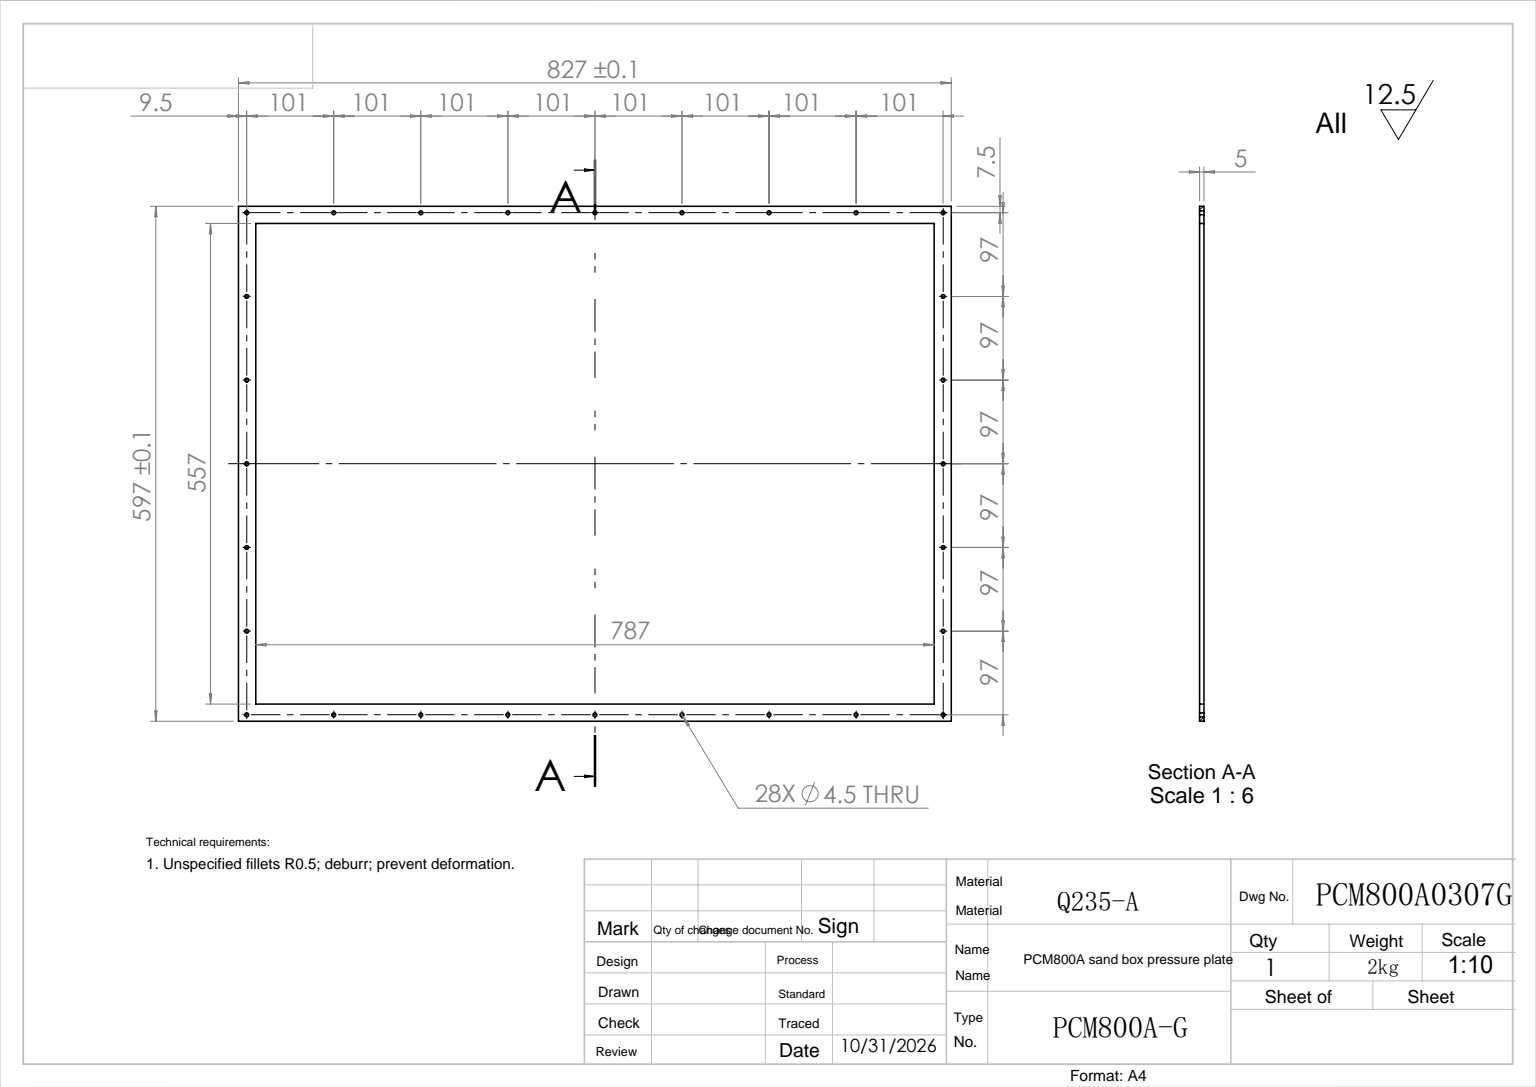
from build123d import *

# Parameters (mm, degrees)
SKETCH_1_W                        = 827
SKETCH_1_H                        = 597
SKETCH_1_W_2                      = 787
SKETCH_1_H_2                      = 557
EXTRUDE_1_DEPTH                   = 5
SKETCH_2_R                        = 2.25
CUT_EXTRUDE_1_DEPTH               = 5
PATTERN_LINEAR_1_COUNT            = 9
PATTERN_LINEAR_1_PITCH            = 101
PATTERN_LINEAR_2_COUNT            = 7
PATTERN_LINEAR_2_PITCH            = 97
PATTERN_LINEAR_3_COPY_1_SKETCH_R  = 2.25
PATTERN_LINEAR_3_COPY_1_DEPTH     = 5
PATTERN_LINEAR_3_COPY_2_SKETCH_R  = 2.25
PATTERN_LINEAR_3_COPY_2_DEPTH     = 5
PATTERN_LINEAR_3_COPY_3_SKETCH_R  = 2.25
PATTERN_LINEAR_3_COPY_3_DEPTH     = 5
PATTERN_LINEAR_3_COPY_4_SKETCH_R  = 2.25
PATTERN_LINEAR_3_COPY_4_DEPTH     = 5
PATTERN_LINEAR_3_COPY_5_SKETCH_R  = 2.25
PATTERN_LINEAR_3_COPY_5_DEPTH     = 5
PATTERN_LINEAR_3_COPY_6_SKETCH_R  = 2.25
PATTERN_LINEAR_3_COPY_6_DEPTH     = 5
PATTERN_LINEAR_3_COPY_7_SKETCH_R  = 2.25
PATTERN_LINEAR_3_COPY_7_DEPTH     = 5
PATTERN_LINEAR_3_COPY_8_SKETCH_R  = 2.25
PATTERN_LINEAR_3_COPY_8_DEPTH     = 5
PATTERN_LINEAR_3_COPY_9_SKETCH_R  = 2.25
PATTERN_LINEAR_3_COPY_9_DEPTH     = 5
PATTERN_LINEAR_3_COPY_10_SKETCH_R = 2.25
PATTERN_LINEAR_3_COPY_10_DEPTH    = 5
PATTERN_LINEAR_3_COPY_11_SKETCH_R = 2.25
PATTERN_LINEAR_3_COPY_11_DEPTH    = 5
PATTERN_LINEAR_3_COPY_12_SKETCH_R = 2.25
PATTERN_LINEAR_3_COPY_12_DEPTH    = 5
PATTERN_LINEAR_3_COPY_13_SKETCH_R = 2.25
PATTERN_LINEAR_3_COPY_13_DEPTH    = 5
PATTERN_LINEAR_3_COPY_14_SKETCH_R = 2.25
PATTERN_LINEAR_3_COPY_14_DEPTH    = 5
PATTERN_LINEAR_3_COPY_15_SKETCH_R = 2.25
PATTERN_LINEAR_3_COPY_15_DEPTH    = 5
PATTERN_LINEAR_3_COPY_16_SKETCH_R = 2.25
PATTERN_LINEAR_3_COPY_16_DEPTH    = 5
PATTERN_LINEAR_3_COPY_17_SKETCH_R = 2.25
PATTERN_LINEAR_3_COPY_17_DEPTH    = 5
PATTERN_LINEAR_3_COPY_18_SKETCH_R = 2.25
PATTERN_LINEAR_3_COPY_18_DEPTH    = 5
PATTERN_LINEAR_3_COPY_19_SKETCH_R = 2.25
PATTERN_LINEAR_3_COPY_19_DEPTH    = 5
PATTERN_LINEAR_3_COPY_20_SKETCH_R = 2.25
PATTERN_LINEAR_3_COPY_20_DEPTH    = 5
PATTERN_LINEAR_3_COPY_21_SKETCH_R = 2.25
PATTERN_LINEAR_3_COPY_21_DEPTH    = 5
PATTERN_LINEAR_3_COPY_22_SKETCH_R = 2.25
PATTERN_LINEAR_3_COPY_22_DEPTH    = 5
PATTERN_LINEAR_3_COPY_23_SKETCH_R = 2.25
PATTERN_LINEAR_3_COPY_23_DEPTH    = 5
PATTERN_LINEAR_3_COPY_24_SKETCH_R = 2.25
PATTERN_LINEAR_3_COPY_24_DEPTH    = 5
PATTERN_LINEAR_3_COPY_25_SKETCH_R = 2.25
PATTERN_LINEAR_3_COPY_25_DEPTH    = 5
PATTERN_LINEAR_3_COPY_26_SKETCH_R = 2.25
PATTERN_LINEAR_3_COPY_26_DEPTH    = 5
PATTERN_LINEAR_3_COPY_27_SKETCH_R = 2.25
PATTERN_LINEAR_3_COPY_27_DEPTH    = 5
PATTERN_LINEAR_3_COPY_28_SKETCH_R = 2.25
PATTERN_LINEAR_3_COPY_28_DEPTH    = 5
PATTERN_LINEAR_3_COPY_29_SKETCH_R = 2.25
PATTERN_LINEAR_3_COPY_29_DEPTH    = 5
PATTERN_LINEAR_3_COPY_30_SKETCH_R = 2.25
PATTERN_LINEAR_3_COPY_30_DEPTH    = 5
PATTERN_LINEAR_3_COPY_31_SKETCH_R = 2.25
PATTERN_LINEAR_3_COPY_31_DEPTH    = 5
PATTERN_LINEAR_3_COPY_32_SKETCH_R = 2.25
PATTERN_LINEAR_3_COPY_32_DEPTH    = 5
PATTERN_LINEAR_3_COPY_33_SKETCH_R = 2.25
PATTERN_LINEAR_3_COPY_33_DEPTH    = 5
PATTERN_LINEAR_3_COPY_34_SKETCH_R = 2.25
PATTERN_LINEAR_3_COPY_34_DEPTH    = 5
PATTERN_LINEAR_3_COPY_35_SKETCH_R = 2.25
PATTERN_LINEAR_3_COPY_35_DEPTH    = 5
PATTERN_LINEAR_3_COPY_36_SKETCH_R = 2.25
PATTERN_LINEAR_3_COPY_36_DEPTH    = 5
PATTERN_LINEAR_3_COPY_37_SKETCH_R = 2.25
PATTERN_LINEAR_3_COPY_37_DEPTH    = 5
PATTERN_LINEAR_3_COPY_38_SKETCH_R = 2.25
PATTERN_LINEAR_3_COPY_38_DEPTH    = 5
PATTERN_LINEAR_3_COPY_39_SKETCH_R = 2.25
PATTERN_LINEAR_3_COPY_39_DEPTH    = 5
PATTERN_LINEAR_3_COPY_40_SKETCH_R = 2.25
PATTERN_LINEAR_3_COPY_40_DEPTH    = 5
PATTERN_LINEAR_3_COPY_41_SKETCH_R = 2.25
PATTERN_LINEAR_3_COPY_41_DEPTH    = 5
PATTERN_LINEAR_3_COPY_42_SKETCH_R = 2.25
PATTERN_LINEAR_3_COPY_42_DEPTH    = 5
PATTERN_LINEAR_3_COPY_43_SKETCH_R = 2.25
PATTERN_LINEAR_3_COPY_43_DEPTH    = 5
PATTERN_LINEAR_3_COPY_44_SKETCH_R = 2.25
PATTERN_LINEAR_3_COPY_44_DEPTH    = 5
PATTERN_LINEAR_3_COPY_45_SKETCH_R = 2.25
PATTERN_LINEAR_3_COPY_45_DEPTH    = 5
PATTERN_LINEAR_3_COPY_46_SKETCH_R = 2.25
PATTERN_LINEAR_3_COPY_46_DEPTH    = 5
PATTERN_LINEAR_3_COPY_47_SKETCH_R = 2.25
PATTERN_LINEAR_3_COPY_47_DEPTH    = 5
PATTERN_LINEAR_3_COPY_48_SKETCH_R = 2.25
PATTERN_LINEAR_3_COPY_48_DEPTH    = 5
PATTERN_LINEAR_3_COPY_49_SKETCH_R = 2.25
PATTERN_LINEAR_3_COPY_49_DEPTH    = 5
PATTERN_LINEAR_3_COPY_50_SKETCH_R = 2.25
PATTERN_LINEAR_3_COPY_50_DEPTH    = 5
PATTERN_LINEAR_3_COPY_51_SKETCH_R = 2.25
PATTERN_LINEAR_3_COPY_51_DEPTH    = 5
PATTERN_LINEAR_3_COPY_52_SKETCH_R = 2.25
PATTERN_LINEAR_3_COPY_52_DEPTH    = 5
PATTERN_LINEAR_3_COPY_53_SKETCH_R = 2.25
PATTERN_LINEAR_3_COPY_53_DEPTH    = 5
PATTERN_LINEAR_3_COPY_54_SKETCH_R = 2.25
PATTERN_LINEAR_3_COPY_54_DEPTH    = 5
PATTERN_LINEAR_3_COPY_55_SKETCH_R = 2.25
PATTERN_LINEAR_3_COPY_55_DEPTH    = 5
PATTERN_LINEAR_3_COPY_56_SKETCH_R = 2.25
PATTERN_LINEAR_3_COPY_56_DEPTH    = 5


with BuildPart() as part:
    # 草图1 → 拉伸1 (new body)
    with BuildSketch(Plane(origin=(0, 0, 0), x_dir=(1, 0, 0), z_dir=(0, 1, 0))):
        with Locations((413.5, 298.5)):
            Rectangle(SKETCH_1_W, SKETCH_1_H)
        with Locations((413.5, 298.5)):
            Rectangle(SKETCH_1_W_2, SKETCH_1_H_2, mode=Mode.SUBTRACT)
    extrude(amount=EXTRUDE_1_DEPTH)

    # 草图2 → 切除-拉伸1 (cut)
    with BuildSketch(Plane(origin=(0, 5, 0), x_dir=(-1, 0, 0), z_dir=(0, 1, 0))):
        with Locations(Location((-817.5, -589.5, 0), (0, 0, 90))):
            Circle(SKETCH_2_R)
    cut_extrude_1 = extrude(amount=-CUT_EXTRUDE_1_DEPTH, mode=Mode.SUBTRACT)

    # 阵列(线性)1: 切除-拉伸1 ×9
    with Locations(*[(-i * PATTERN_LINEAR_1_PITCH, 0, 0) for i in range(1, PATTERN_LINEAR_1_COUNT)]):
        add(cut_extrude_1, mode=Mode.SUBTRACT)

    # 阵列(线性)2: 切除-拉伸1 ×7
    with Locations(*[(0, 0, i * PATTERN_LINEAR_2_PITCH) for i in range(1, PATTERN_LINEAR_2_COUNT)]):
        add(cut_extrude_1, mode=Mode.SUBTRACT)

    # 阵列(线性)3 copy 1 sketch → 阵列(线性)3 copy 1 (cut)
    with BuildSketch(Plane(origin=(-101, 5, 97), x_dir=(-1, 0, 0), z_dir=(0, 1, 0))):
        with Locations(Location((-817.5, -589.5, 0), (0, 0, 90))):
            Circle(PATTERN_LINEAR_3_COPY_1_SKETCH_R)
    extrude(amount=-PATTERN_LINEAR_3_COPY_1_DEPTH, mode=Mode.SUBTRACT)

    # 阵列(线性)3 copy 2 sketch → 阵列(线性)3 copy 2 (cut)
    with BuildSketch(Plane(origin=(-202, 5, 97), x_dir=(-1, 0, 0), z_dir=(0, 1, 0))):
        with Locations(Location((-817.5, -589.5, 0), (0, 0, 90))):
            Circle(PATTERN_LINEAR_3_COPY_2_SKETCH_R)
    extrude(amount=-PATTERN_LINEAR_3_COPY_2_DEPTH, mode=Mode.SUBTRACT)

    # 阵列(线性)3 copy 3 sketch → 阵列(线性)3 copy 3 (cut)
    with BuildSketch(Plane(origin=(-303, 5, 97), x_dir=(-1, 0, 0), z_dir=(0, 1, 0))):
        with Locations(Location((-817.5, -589.5, 0), (0, 0, 90))):
            Circle(PATTERN_LINEAR_3_COPY_3_SKETCH_R)
    extrude(amount=-PATTERN_LINEAR_3_COPY_3_DEPTH, mode=Mode.SUBTRACT)

    # 阵列(线性)3 copy 4 sketch → 阵列(线性)3 copy 4 (cut)
    with BuildSketch(Plane(origin=(-404, 5, 97), x_dir=(-1, 0, 0), z_dir=(0, 1, 0))):
        with Locations(Location((-817.5, -589.5, 0), (0, 0, 90))):
            Circle(PATTERN_LINEAR_3_COPY_4_SKETCH_R)
    extrude(amount=-PATTERN_LINEAR_3_COPY_4_DEPTH, mode=Mode.SUBTRACT)

    # 阵列(线性)3 copy 5 sketch → 阵列(线性)3 copy 5 (cut)
    with BuildSketch(Plane(origin=(-505, 5, 97), x_dir=(-1, 0, 0), z_dir=(0, 1, 0))):
        with Locations(Location((-817.5, -589.5, 0), (0, 0, 90))):
            Circle(PATTERN_LINEAR_3_COPY_5_SKETCH_R)
    extrude(amount=-PATTERN_LINEAR_3_COPY_5_DEPTH, mode=Mode.SUBTRACT)

    # 阵列(线性)3 copy 6 sketch → 阵列(线性)3 copy 6 (cut)
    with BuildSketch(Plane(origin=(-606, 5, 97), x_dir=(-1, 0, 0), z_dir=(0, 1, 0))):
        with Locations(Location((-817.5, -589.5, 0), (0, 0, 90))):
            Circle(PATTERN_LINEAR_3_COPY_6_SKETCH_R)
    extrude(amount=-PATTERN_LINEAR_3_COPY_6_DEPTH, mode=Mode.SUBTRACT)

    # 阵列(线性)3 copy 7 sketch → 阵列(线性)3 copy 7 (cut)
    with BuildSketch(Plane(origin=(-707, 5, 97), x_dir=(-1, 0, 0), z_dir=(0, 1, 0))):
        with Locations(Location((-817.5, -589.5, 0), (0, 0, 90))):
            Circle(PATTERN_LINEAR_3_COPY_7_SKETCH_R)
    extrude(amount=-PATTERN_LINEAR_3_COPY_7_DEPTH, mode=Mode.SUBTRACT)

    # 阵列(线性)3 copy 8 sketch → 阵列(线性)3 copy 8 (cut)
    with BuildSketch(Plane(origin=(-808, 5, 97), x_dir=(-1, 0, 0), z_dir=(0, 1, 0))):
        with Locations(Location((-817.5, -589.5, 0), (0, 0, 90))):
            Circle(PATTERN_LINEAR_3_COPY_8_SKETCH_R)
    extrude(amount=-PATTERN_LINEAR_3_COPY_8_DEPTH, mode=Mode.SUBTRACT)

    # 阵列(线性)3 copy 9 sketch → 阵列(线性)3 copy 9 (cut)
    with BuildSketch(Plane(origin=(-101, 5, 194), x_dir=(-1, 0, 0), z_dir=(0, 1, 0))):
        with Locations(Location((-817.5, -589.5, 0), (0, 0, 90))):
            Circle(PATTERN_LINEAR_3_COPY_9_SKETCH_R)
    extrude(amount=-PATTERN_LINEAR_3_COPY_9_DEPTH, mode=Mode.SUBTRACT)

    # 阵列(线性)3 copy 10 sketch → 阵列(线性)3 copy 10 (cut)
    with BuildSketch(Plane(origin=(-202, 5, 194), x_dir=(-1, 0, 0), z_dir=(0, 1, 0))):
        with Locations(Location((-817.5, -589.5, 0), (0, 0, 90))):
            Circle(PATTERN_LINEAR_3_COPY_10_SKETCH_R)
    extrude(amount=-PATTERN_LINEAR_3_COPY_10_DEPTH, mode=Mode.SUBTRACT)

    # 阵列(线性)3 copy 11 sketch → 阵列(线性)3 copy 11 (cut)
    with BuildSketch(Plane(origin=(-303, 5, 194), x_dir=(-1, 0, 0), z_dir=(0, 1, 0))):
        with Locations(Location((-817.5, -589.5, 0), (0, 0, 90))):
            Circle(PATTERN_LINEAR_3_COPY_11_SKETCH_R)
    extrude(amount=-PATTERN_LINEAR_3_COPY_11_DEPTH, mode=Mode.SUBTRACT)

    # 阵列(线性)3 copy 12 sketch → 阵列(线性)3 copy 12 (cut)
    with BuildSketch(Plane(origin=(-404, 5, 194), x_dir=(-1, 0, 0), z_dir=(0, 1, 0))):
        with Locations(Location((-817.5, -589.5, 0), (0, 0, 90))):
            Circle(PATTERN_LINEAR_3_COPY_12_SKETCH_R)
    extrude(amount=-PATTERN_LINEAR_3_COPY_12_DEPTH, mode=Mode.SUBTRACT)

    # 阵列(线性)3 copy 13 sketch → 阵列(线性)3 copy 13 (cut)
    with BuildSketch(Plane(origin=(-505, 5, 194), x_dir=(-1, 0, 0), z_dir=(0, 1, 0))):
        with Locations(Location((-817.5, -589.5, 0), (0, 0, 90))):
            Circle(PATTERN_LINEAR_3_COPY_13_SKETCH_R)
    extrude(amount=-PATTERN_LINEAR_3_COPY_13_DEPTH, mode=Mode.SUBTRACT)

    # 阵列(线性)3 copy 14 sketch → 阵列(线性)3 copy 14 (cut)
    with BuildSketch(Plane(origin=(-606, 5, 194), x_dir=(-1, 0, 0), z_dir=(0, 1, 0))):
        with Locations(Location((-817.5, -589.5, 0), (0, 0, 90))):
            Circle(PATTERN_LINEAR_3_COPY_14_SKETCH_R)
    extrude(amount=-PATTERN_LINEAR_3_COPY_14_DEPTH, mode=Mode.SUBTRACT)

    # 阵列(线性)3 copy 15 sketch → 阵列(线性)3 copy 15 (cut)
    with BuildSketch(Plane(origin=(-707, 5, 194), x_dir=(-1, 0, 0), z_dir=(0, 1, 0))):
        with Locations(Location((-817.5, -589.5, 0), (0, 0, 90))):
            Circle(PATTERN_LINEAR_3_COPY_15_SKETCH_R)
    extrude(amount=-PATTERN_LINEAR_3_COPY_15_DEPTH, mode=Mode.SUBTRACT)

    # 阵列(线性)3 copy 16 sketch → 阵列(线性)3 copy 16 (cut)
    with BuildSketch(Plane(origin=(-808, 5, 194), x_dir=(-1, 0, 0), z_dir=(0, 1, 0))):
        with Locations(Location((-817.5, -589.5, 0), (0, 0, 90))):
            Circle(PATTERN_LINEAR_3_COPY_16_SKETCH_R)
    extrude(amount=-PATTERN_LINEAR_3_COPY_16_DEPTH, mode=Mode.SUBTRACT)

    # 阵列(线性)3 copy 17 sketch → 阵列(线性)3 copy 17 (cut)
    with BuildSketch(Plane(origin=(-101, 5, 291), x_dir=(-1, 0, 0), z_dir=(0, 1, 0))):
        with Locations(Location((-817.5, -589.5, 0), (0, 0, 90))):
            Circle(PATTERN_LINEAR_3_COPY_17_SKETCH_R)
    extrude(amount=-PATTERN_LINEAR_3_COPY_17_DEPTH, mode=Mode.SUBTRACT)

    # 阵列(线性)3 copy 18 sketch → 阵列(线性)3 copy 18 (cut)
    with BuildSketch(Plane(origin=(-202, 5, 291), x_dir=(-1, 0, 0), z_dir=(0, 1, 0))):
        with Locations(Location((-817.5, -589.5, 0), (0, 0, 90))):
            Circle(PATTERN_LINEAR_3_COPY_18_SKETCH_R)
    extrude(amount=-PATTERN_LINEAR_3_COPY_18_DEPTH, mode=Mode.SUBTRACT)

    # 阵列(线性)3 copy 19 sketch → 阵列(线性)3 copy 19 (cut)
    with BuildSketch(Plane(origin=(-303, 5, 291), x_dir=(-1, 0, 0), z_dir=(0, 1, 0))):
        with Locations(Location((-817.5, -589.5, 0), (0, 0, 90))):
            Circle(PATTERN_LINEAR_3_COPY_19_SKETCH_R)
    extrude(amount=-PATTERN_LINEAR_3_COPY_19_DEPTH, mode=Mode.SUBTRACT)

    # 阵列(线性)3 copy 20 sketch → 阵列(线性)3 copy 20 (cut)
    with BuildSketch(Plane(origin=(-404, 5, 291), x_dir=(-1, 0, 0), z_dir=(0, 1, 0))):
        with Locations(Location((-817.5, -589.5, 0), (0, 0, 90))):
            Circle(PATTERN_LINEAR_3_COPY_20_SKETCH_R)
    extrude(amount=-PATTERN_LINEAR_3_COPY_20_DEPTH, mode=Mode.SUBTRACT)

    # 阵列(线性)3 copy 21 sketch → 阵列(线性)3 copy 21 (cut)
    with BuildSketch(Plane(origin=(-505, 5, 291), x_dir=(-1, 0, 0), z_dir=(0, 1, 0))):
        with Locations(Location((-817.5, -589.5, 0), (0, 0, 90))):
            Circle(PATTERN_LINEAR_3_COPY_21_SKETCH_R)
    extrude(amount=-PATTERN_LINEAR_3_COPY_21_DEPTH, mode=Mode.SUBTRACT)

    # 阵列(线性)3 copy 22 sketch → 阵列(线性)3 copy 22 (cut)
    with BuildSketch(Plane(origin=(-606, 5, 291), x_dir=(-1, 0, 0), z_dir=(0, 1, 0))):
        with Locations(Location((-817.5, -589.5, 0), (0, 0, 90))):
            Circle(PATTERN_LINEAR_3_COPY_22_SKETCH_R)
    extrude(amount=-PATTERN_LINEAR_3_COPY_22_DEPTH, mode=Mode.SUBTRACT)

    # 阵列(线性)3 copy 23 sketch → 阵列(线性)3 copy 23 (cut)
    with BuildSketch(Plane(origin=(-707, 5, 291), x_dir=(-1, 0, 0), z_dir=(0, 1, 0))):
        with Locations(Location((-817.5, -589.5, 0), (0, 0, 90))):
            Circle(PATTERN_LINEAR_3_COPY_23_SKETCH_R)
    extrude(amount=-PATTERN_LINEAR_3_COPY_23_DEPTH, mode=Mode.SUBTRACT)

    # 阵列(线性)3 copy 24 sketch → 阵列(线性)3 copy 24 (cut)
    with BuildSketch(Plane(origin=(-808, 5, 291), x_dir=(-1, 0, 0), z_dir=(0, 1, 0))):
        with Locations(Location((-817.5, -589.5, 0), (0, 0, 90))):
            Circle(PATTERN_LINEAR_3_COPY_24_SKETCH_R)
    extrude(amount=-PATTERN_LINEAR_3_COPY_24_DEPTH, mode=Mode.SUBTRACT)

    # 阵列(线性)3 copy 25 sketch → 阵列(线性)3 copy 25 (cut)
    with BuildSketch(Plane(origin=(-101, 5, 388), x_dir=(-1, 0, 0), z_dir=(0, 1, 0))):
        with Locations(Location((-817.5, -589.5, 0), (0, 0, 90))):
            Circle(PATTERN_LINEAR_3_COPY_25_SKETCH_R)
    extrude(amount=-PATTERN_LINEAR_3_COPY_25_DEPTH, mode=Mode.SUBTRACT)

    # 阵列(线性)3 copy 26 sketch → 阵列(线性)3 copy 26 (cut)
    with BuildSketch(Plane(origin=(-202, 5, 388), x_dir=(-1, 0, 0), z_dir=(0, 1, 0))):
        with Locations(Location((-817.5, -589.5, 0), (0, 0, 90))):
            Circle(PATTERN_LINEAR_3_COPY_26_SKETCH_R)
    extrude(amount=-PATTERN_LINEAR_3_COPY_26_DEPTH, mode=Mode.SUBTRACT)

    # 阵列(线性)3 copy 27 sketch → 阵列(线性)3 copy 27 (cut)
    with BuildSketch(Plane(origin=(-303, 5, 388), x_dir=(-1, 0, 0), z_dir=(0, 1, 0))):
        with Locations(Location((-817.5, -589.5, 0), (0, 0, 90))):
            Circle(PATTERN_LINEAR_3_COPY_27_SKETCH_R)
    extrude(amount=-PATTERN_LINEAR_3_COPY_27_DEPTH, mode=Mode.SUBTRACT)

    # 阵列(线性)3 copy 28 sketch → 阵列(线性)3 copy 28 (cut)
    with BuildSketch(Plane(origin=(-404, 5, 388), x_dir=(-1, 0, 0), z_dir=(0, 1, 0))):
        with Locations(Location((-817.5, -589.5, 0), (0, 0, 90))):
            Circle(PATTERN_LINEAR_3_COPY_28_SKETCH_R)
    extrude(amount=-PATTERN_LINEAR_3_COPY_28_DEPTH, mode=Mode.SUBTRACT)

    # 阵列(线性)3 copy 29 sketch → 阵列(线性)3 copy 29 (cut)
    with BuildSketch(Plane(origin=(-505, 5, 388), x_dir=(-1, 0, 0), z_dir=(0, 1, 0))):
        with Locations(Location((-817.5, -589.5, 0), (0, 0, 90))):
            Circle(PATTERN_LINEAR_3_COPY_29_SKETCH_R)
    extrude(amount=-PATTERN_LINEAR_3_COPY_29_DEPTH, mode=Mode.SUBTRACT)

    # 阵列(线性)3 copy 30 sketch → 阵列(线性)3 copy 30 (cut)
    with BuildSketch(Plane(origin=(-606, 5, 388), x_dir=(-1, 0, 0), z_dir=(0, 1, 0))):
        with Locations(Location((-817.5, -589.5, 0), (0, 0, 90))):
            Circle(PATTERN_LINEAR_3_COPY_30_SKETCH_R)
    extrude(amount=-PATTERN_LINEAR_3_COPY_30_DEPTH, mode=Mode.SUBTRACT)

    # 阵列(线性)3 copy 31 sketch → 阵列(线性)3 copy 31 (cut)
    with BuildSketch(Plane(origin=(-707, 5, 388), x_dir=(-1, 0, 0), z_dir=(0, 1, 0))):
        with Locations(Location((-817.5, -589.5, 0), (0, 0, 90))):
            Circle(PATTERN_LINEAR_3_COPY_31_SKETCH_R)
    extrude(amount=-PATTERN_LINEAR_3_COPY_31_DEPTH, mode=Mode.SUBTRACT)

    # 阵列(线性)3 copy 32 sketch → 阵列(线性)3 copy 32 (cut)
    with BuildSketch(Plane(origin=(-808, 5, 388), x_dir=(-1, 0, 0), z_dir=(0, 1, 0))):
        with Locations(Location((-817.5, -589.5, 0), (0, 0, 90))):
            Circle(PATTERN_LINEAR_3_COPY_32_SKETCH_R)
    extrude(amount=-PATTERN_LINEAR_3_COPY_32_DEPTH, mode=Mode.SUBTRACT)

    # 阵列(线性)3 copy 33 sketch → 阵列(线性)3 copy 33 (cut)
    with BuildSketch(Plane(origin=(-101, 5, 485), x_dir=(-1, 0, 0), z_dir=(0, 1, 0))):
        with Locations(Location((-817.5, -589.5, 0), (0, 0, 90))):
            Circle(PATTERN_LINEAR_3_COPY_33_SKETCH_R)
    extrude(amount=-PATTERN_LINEAR_3_COPY_33_DEPTH, mode=Mode.SUBTRACT)

    # 阵列(线性)3 copy 34 sketch → 阵列(线性)3 copy 34 (cut)
    with BuildSketch(Plane(origin=(-202, 5, 485), x_dir=(-1, 0, 0), z_dir=(0, 1, 0))):
        with Locations(Location((-817.5, -589.5, 0), (0, 0, 90))):
            Circle(PATTERN_LINEAR_3_COPY_34_SKETCH_R)
    extrude(amount=-PATTERN_LINEAR_3_COPY_34_DEPTH, mode=Mode.SUBTRACT)

    # 阵列(线性)3 copy 35 sketch → 阵列(线性)3 copy 35 (cut)
    with BuildSketch(Plane(origin=(-303, 5, 485), x_dir=(-1, 0, 0), z_dir=(0, 1, 0))):
        with Locations(Location((-817.5, -589.5, 0), (0, 0, 90))):
            Circle(PATTERN_LINEAR_3_COPY_35_SKETCH_R)
    extrude(amount=-PATTERN_LINEAR_3_COPY_35_DEPTH, mode=Mode.SUBTRACT)

    # 阵列(线性)3 copy 36 sketch → 阵列(线性)3 copy 36 (cut)
    with BuildSketch(Plane(origin=(-404, 5, 485), x_dir=(-1, 0, 0), z_dir=(0, 1, 0))):
        with Locations(Location((-817.5, -589.5, 0), (0, 0, 90))):
            Circle(PATTERN_LINEAR_3_COPY_36_SKETCH_R)
    extrude(amount=-PATTERN_LINEAR_3_COPY_36_DEPTH, mode=Mode.SUBTRACT)

    # 阵列(线性)3 copy 37 sketch → 阵列(线性)3 copy 37 (cut)
    with BuildSketch(Plane(origin=(-505, 5, 485), x_dir=(-1, 0, 0), z_dir=(0, 1, 0))):
        with Locations(Location((-817.5, -589.5, 0), (0, 0, 90))):
            Circle(PATTERN_LINEAR_3_COPY_37_SKETCH_R)
    extrude(amount=-PATTERN_LINEAR_3_COPY_37_DEPTH, mode=Mode.SUBTRACT)

    # 阵列(线性)3 copy 38 sketch → 阵列(线性)3 copy 38 (cut)
    with BuildSketch(Plane(origin=(-606, 5, 485), x_dir=(-1, 0, 0), z_dir=(0, 1, 0))):
        with Locations(Location((-817.5, -589.5, 0), (0, 0, 90))):
            Circle(PATTERN_LINEAR_3_COPY_38_SKETCH_R)
    extrude(amount=-PATTERN_LINEAR_3_COPY_38_DEPTH, mode=Mode.SUBTRACT)

    # 阵列(线性)3 copy 39 sketch → 阵列(线性)3 copy 39 (cut)
    with BuildSketch(Plane(origin=(-707, 5, 485), x_dir=(-1, 0, 0), z_dir=(0, 1, 0))):
        with Locations(Location((-817.5, -589.5, 0), (0, 0, 90))):
            Circle(PATTERN_LINEAR_3_COPY_39_SKETCH_R)
    extrude(amount=-PATTERN_LINEAR_3_COPY_39_DEPTH, mode=Mode.SUBTRACT)

    # 阵列(线性)3 copy 40 sketch → 阵列(线性)3 copy 40 (cut)
    with BuildSketch(Plane(origin=(-808, 5, 485), x_dir=(-1, 0, 0), z_dir=(0, 1, 0))):
        with Locations(Location((-817.5, -589.5, 0), (0, 0, 90))):
            Circle(PATTERN_LINEAR_3_COPY_40_SKETCH_R)
    extrude(amount=-PATTERN_LINEAR_3_COPY_40_DEPTH, mode=Mode.SUBTRACT)

    # 阵列(线性)3 copy 41 sketch → 阵列(线性)3 copy 41 (cut)
    with BuildSketch(Plane(origin=(-101, 5, 582), x_dir=(-1, 0, 0), z_dir=(0, 1, 0))):
        with Locations(Location((-817.5, -589.5, 0), (0, 0, 90))):
            Circle(PATTERN_LINEAR_3_COPY_41_SKETCH_R)
    extrude(amount=-PATTERN_LINEAR_3_COPY_41_DEPTH, mode=Mode.SUBTRACT)

    # 阵列(线性)3 copy 42 sketch → 阵列(线性)3 copy 42 (cut)
    with BuildSketch(Plane(origin=(-202, 5, 582), x_dir=(-1, 0, 0), z_dir=(0, 1, 0))):
        with Locations(Location((-817.5, -589.5, 0), (0, 0, 90))):
            Circle(PATTERN_LINEAR_3_COPY_42_SKETCH_R)
    extrude(amount=-PATTERN_LINEAR_3_COPY_42_DEPTH, mode=Mode.SUBTRACT)

    # 阵列(线性)3 copy 43 sketch → 阵列(线性)3 copy 43 (cut)
    with BuildSketch(Plane(origin=(-303, 5, 582), x_dir=(-1, 0, 0), z_dir=(0, 1, 0))):
        with Locations(Location((-817.5, -589.5, 0), (0, 0, 90))):
            Circle(PATTERN_LINEAR_3_COPY_43_SKETCH_R)
    extrude(amount=-PATTERN_LINEAR_3_COPY_43_DEPTH, mode=Mode.SUBTRACT)

    # 阵列(线性)3 copy 44 sketch → 阵列(线性)3 copy 44 (cut)
    with BuildSketch(Plane(origin=(-404, 5, 582), x_dir=(-1, 0, 0), z_dir=(0, 1, 0))):
        with Locations(Location((-817.5, -589.5, 0), (0, 0, 90))):
            Circle(PATTERN_LINEAR_3_COPY_44_SKETCH_R)
    extrude(amount=-PATTERN_LINEAR_3_COPY_44_DEPTH, mode=Mode.SUBTRACT)

    # 阵列(线性)3 copy 45 sketch → 阵列(线性)3 copy 45 (cut)
    with BuildSketch(Plane(origin=(-505, 5, 582), x_dir=(-1, 0, 0), z_dir=(0, 1, 0))):
        with Locations(Location((-817.5, -589.5, 0), (0, 0, 90))):
            Circle(PATTERN_LINEAR_3_COPY_45_SKETCH_R)
    extrude(amount=-PATTERN_LINEAR_3_COPY_45_DEPTH, mode=Mode.SUBTRACT)

    # 阵列(线性)3 copy 46 sketch → 阵列(线性)3 copy 46 (cut)
    with BuildSketch(Plane(origin=(-606, 5, 582), x_dir=(-1, 0, 0), z_dir=(0, 1, 0))):
        with Locations(Location((-817.5, -589.5, 0), (0, 0, 90))):
            Circle(PATTERN_LINEAR_3_COPY_46_SKETCH_R)
    extrude(amount=-PATTERN_LINEAR_3_COPY_46_DEPTH, mode=Mode.SUBTRACT)

    # 阵列(线性)3 copy 47 sketch → 阵列(线性)3 copy 47 (cut)
    with BuildSketch(Plane(origin=(-707, 5, 582), x_dir=(-1, 0, 0), z_dir=(0, 1, 0))):
        with Locations(Location((-817.5, -589.5, 0), (0, 0, 90))):
            Circle(PATTERN_LINEAR_3_COPY_47_SKETCH_R)
    extrude(amount=-PATTERN_LINEAR_3_COPY_47_DEPTH, mode=Mode.SUBTRACT)

    # 阵列(线性)3 copy 48 sketch → 阵列(线性)3 copy 48 (cut)
    with BuildSketch(Plane(origin=(-808, 5, 582), x_dir=(-1, 0, 0), z_dir=(0, 1, 0))):
        with Locations(Location((-817.5, -589.5, 0), (0, 0, 90))):
            Circle(PATTERN_LINEAR_3_COPY_48_SKETCH_R)
    extrude(amount=-PATTERN_LINEAR_3_COPY_48_DEPTH, mode=Mode.SUBTRACT)

    # 阵列(线性)3 copy 49 sketch → 阵列(线性)3 copy 49 (cut)
    with BuildSketch(Plane(origin=(-101, 5, 0), x_dir=(-1, 0, 0), z_dir=(0, 1, 0))):
        with Locations(Location((-817.5, -589.5, 0), (0, 0, 90))):
            Circle(PATTERN_LINEAR_3_COPY_49_SKETCH_R)
    extrude(amount=-PATTERN_LINEAR_3_COPY_49_DEPTH, mode=Mode.SUBTRACT)

    # 阵列(线性)3 copy 50 sketch → 阵列(线性)3 copy 50 (cut)
    with BuildSketch(Plane(origin=(-202, 5, 0), x_dir=(-1, 0, 0), z_dir=(0, 1, 0))):
        with Locations(Location((-817.5, -589.5, 0), (0, 0, 90))):
            Circle(PATTERN_LINEAR_3_COPY_50_SKETCH_R)
    extrude(amount=-PATTERN_LINEAR_3_COPY_50_DEPTH, mode=Mode.SUBTRACT)

    # 阵列(线性)3 copy 51 sketch → 阵列(线性)3 copy 51 (cut)
    with BuildSketch(Plane(origin=(-303, 5, 0), x_dir=(-1, 0, 0), z_dir=(0, 1, 0))):
        with Locations(Location((-817.5, -589.5, 0), (0, 0, 90))):
            Circle(PATTERN_LINEAR_3_COPY_51_SKETCH_R)
    extrude(amount=-PATTERN_LINEAR_3_COPY_51_DEPTH, mode=Mode.SUBTRACT)

    # 阵列(线性)3 copy 52 sketch → 阵列(线性)3 copy 52 (cut)
    with BuildSketch(Plane(origin=(-404, 5, 0), x_dir=(-1, 0, 0), z_dir=(0, 1, 0))):
        with Locations(Location((-817.5, -589.5, 0), (0, 0, 90))):
            Circle(PATTERN_LINEAR_3_COPY_52_SKETCH_R)
    extrude(amount=-PATTERN_LINEAR_3_COPY_52_DEPTH, mode=Mode.SUBTRACT)

    # 阵列(线性)3 copy 53 sketch → 阵列(线性)3 copy 53 (cut)
    with BuildSketch(Plane(origin=(-505, 5, 0), x_dir=(-1, 0, 0), z_dir=(0, 1, 0))):
        with Locations(Location((-817.5, -589.5, 0), (0, 0, 90))):
            Circle(PATTERN_LINEAR_3_COPY_53_SKETCH_R)
    extrude(amount=-PATTERN_LINEAR_3_COPY_53_DEPTH, mode=Mode.SUBTRACT)

    # 阵列(线性)3 copy 54 sketch → 阵列(线性)3 copy 54 (cut)
    with BuildSketch(Plane(origin=(-606, 5, 0), x_dir=(-1, 0, 0), z_dir=(0, 1, 0))):
        with Locations(Location((-817.5, -589.5, 0), (0, 0, 90))):
            Circle(PATTERN_LINEAR_3_COPY_54_SKETCH_R)
    extrude(amount=-PATTERN_LINEAR_3_COPY_54_DEPTH, mode=Mode.SUBTRACT)

    # 阵列(线性)3 copy 55 sketch → 阵列(线性)3 copy 55 (cut)
    with BuildSketch(Plane(origin=(-707, 5, 0), x_dir=(-1, 0, 0), z_dir=(0, 1, 0))):
        with Locations(Location((-817.5, -589.5, 0), (0, 0, 90))):
            Circle(PATTERN_LINEAR_3_COPY_55_SKETCH_R)
    extrude(amount=-PATTERN_LINEAR_3_COPY_55_DEPTH, mode=Mode.SUBTRACT)

    # 阵列(线性)3 copy 56 sketch → 阵列(线性)3 copy 56 (cut)
    with BuildSketch(Plane(origin=(-808, 5, 0), x_dir=(-1, 0, 0), z_dir=(0, 1, 0))):
        with Locations(Location((-817.5, -589.5, 0), (0, 0, 90))):
            Circle(PATTERN_LINEAR_3_COPY_56_SKETCH_R)
    extrude(amount=-PATTERN_LINEAR_3_COPY_56_DEPTH, mode=Mode.SUBTRACT)


solid = part.part
